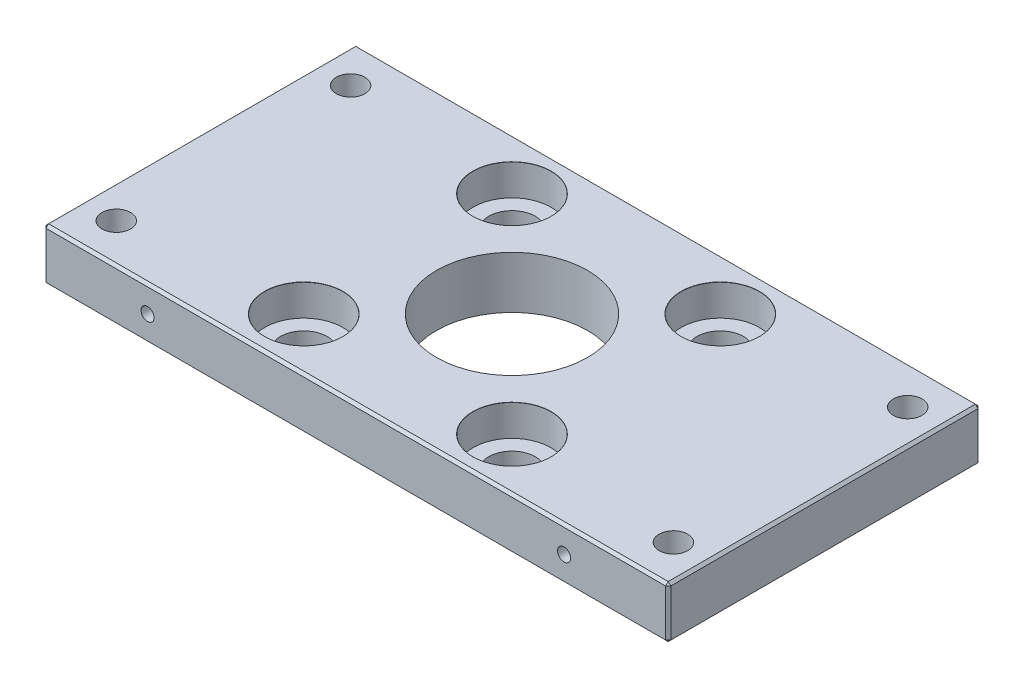
SolidWorks part; units mm, degrees
ref_plane "Front Plane" through (0, 0, 0) normal (0, 0, 1) x (1, 0, 0)
ref_plane "Top Plane" through (0, 0, 0) normal (0, 1, 0) x (1, 0, 0)
ref_plane "Right Plane" through (0, 0, 0) normal (1, 0, 0) x (0, 0, -1)
other "Configuration Table"
sketch "Sketch1" plane through (0, 0, 0) normal (0, 1, 0) x (1, 0, 0)
  line L1 (0, 0) -> (120, 0)
  line L2 (0, 0) -> (0, 60)
  line L3 (0, 60) -> (120, 60)
  line L4 (120, 0) -> (120, 60)
  dimension "D1" = 120
  dimension "D2" = 60
extrude "Boss-Extrude1" add sketch "Sketch1" along normal blind 10
sketch "Sketch2" plane through (0, 10, 0) normal (0, 1, 0) x (1, 0, 0)
  line L0 (0, 30) -> (120, 30) construction
  line L1 (0, 60) -> (0, 0) construction
  line L2 (120, 0) -> (120, 60) construction
  line L3 (60, 60) -> (60, 0) construction
  line L4 (120, 60) -> (0, 60) construction
  line L5 (0, 0) -> (120, 0) construction
  circle A0 centre (60, 30) radius 14.5
  dimension "D1" = 29
extrude "Cut-Extrude1" cut sketch "Sketch2" against normal blind 10
sketch "Sketch4" plane through (0, 10, 0) normal (0, 1, 0) x (1, 0, 0)
  line L0 (60, 60) -> (60, 0) construction
  line L1 (120, 60) -> (0, 60) construction
  line L2 (0, 0) -> (120, 0) construction
  line L3 (0, 30) -> (120, 30) construction
  line L4 (0, 60) -> (0, 0) construction
  line L5 (120, 0) -> (120, 60) construction
  point P16 (40, 50)
  point P17 (80, 50)
  point P21 (40, 10)
  point P22 (80, 10)
  dimension "D1" = 40
  dimension "D2" = 20
  dimension "D3" = 40
  dimension "D4" = 20
  dimension "D5" = 20
  dimension "D6" = 20
  dimension "D7" = 20
  dimension "D8" = 20
hole_wizard "CBORE for M8 Slotted cheese head screws1" positions "Sketch4" profile "Sketch5" counterbore size "M8" standard "GB" end condition through all
sketch "Sketch5" plane through (80, 10, -10) normal (1, 0, 0) x (0, 0, 1)
  line L0 (0, 0) -> (0, 10)
  line L1 (0, 10) -> (4.5, 10)
  line L3 (4.5, 10) -> (4.5, 6)
  line L4 (7.5, 6) -> (4.5, 6)
  line L5 (7.5, 6) -> (7.5, 0.025)
  line L6 (7.5, 0.025) -> (7.525, 0)
  line L7 (7.525, 0) -> (0, 0)
  line L8 (-7.5, 0.025) -> (-7.525, 0) construction
  line L11 (0, -6.35) -> (0, 107.95) construction
  dimension "通孔孔直径" = 9
  dimension "通孔孔深度" = 10
  dimension "柱形沉头孔直径" = 15
  dimension "柱形沉头孔深度" = 6
  dimension "近端锥形沉头孔直径" = 15.05
  dimension "近端锥形沉头孔角度" = 90
sketch "Sketch6" plane through (0, 0, 0) normal (0, -1, 0) x (1, 0, 0)
  line L0 (0, -60) -> (0, 0) construction
  line L1 (0, 0) -> (120, 0) construction
  line L2 (6.5, -7.5) -> (6.5, -52.5) construction
  line L3 (120, 0) -> (120, -60) construction
  line L4 (113.5, -7.5) -> (113.5, -52.5) construction
  point P0 (6.5, -7.5)
  point P5 (6.5, -52.5)
  point P7 (113.5, -7.5)
  point P13 (113.5, -52.5)
  dimension "D1" = 6.5
  dimension "D2" = 7.5
  dimension "D4" = 45
  dimension "D5" = 6.5
  dimension "D7" = 45
  dimension "D8" = 107
  dimension "D3" = 2
  dimension "D6" = 2
hole_wizard "CBORE for M5 Slotted cheese head screws1" positions "Sketch6" profile "Sketch7" counterbore size "M5" standard "GB" end condition through all
sketch "Sketch7" plane through (6.5, 0, -7.5) normal (1, 0, 0) x (0, 0, -1)
  line L0 (0, 0) -> (0, 10)
  line L1 (0, 10) -> (2.75, 10)
  line L3 (2.75, 10) -> (2.75, 5.7)
  line L4 (5, 5.7) -> (2.75, 5.7)
  line L5 (5, 5.7) -> (5, 0.025)
  line L6 (5, 0.025) -> (5.025, 0)
  line L7 (5.025, 0) -> (0, 0)
  line L8 (-5, 0.025) -> (-5.025, 0) construction
  line L11 (0, -6.35) -> (0, 107.95) construction
  dimension "通孔孔直径" = 5.5
  dimension "通孔孔深度" = 10
  dimension "柱形沉头孔直径" = 10
  dimension "柱形沉头孔深度" = 5.7
  dimension "近端锥形沉头孔直径" = 10.05
  dimension "近端锥形沉头孔角度" = 90
sketch "Sketch8" plane through (0, 0, 0) normal (0, -1, 0) x (1, 0, 0)
  line L0 (40, -10) -> (80, -50) construction
  line L1 (80, -10) -> (40, -50) construction
  circle A0 centre (43.182, -13.182) radius 2.5
  circle A1 centre (40, -10) radius 4.5 construction
  circle A2 centre (76.818, -13.182) radius 2.5
  circle A3 centre (80, -10) radius 4.5 construction
  circle A4 centre (76.818, -46.818) radius 2.5
  circle A5 centre (80, -50) radius 4.5 construction
  circle A6 centre (43.182, -46.818) radius 2.5
  circle A7 centre (40, -50) radius 4.5 construction
  dimension "D1" = 5
  dimension "D2" = 5
  dimension "D3" = 5
  dimension "D4" = 5
extrude "Cut-Extrude2" [suppressed] cut sketch "Sketch8" against normal blind 10
sketch "Sketch10" plane through (0, 0, 0) normal (0, 0, 1) x (1, 0, 0)
  line L0 (0, 10) -> (0, 0) construction
  line L1 (0, 10) -> (120, 10) construction
  line L2 (120, 10) -> (120, 0) construction
  point P0 (20, 5)
  point P1 (100, 5)
  dimension "D1" = 20
  dimension "D2" = 5
  dimension "D3" = 20
hole_wizard "M3 Tapped Hole1" positions "Sketch10" profile "Sketch11" tap size "M3" standard "GB"
sketch "Sketch11" plane through (20, 5, 0) normal (1, 0, 0) x (0, -1, 0)
  line L0 (0, 0) -> (0, 12.7511)
  line L1 (0, 12.7511) -> (1.25, 12)
  line L2 (1.25, 12) -> (1.25, 0)
  line L5 (1.25, 0) -> (0, 0)
  line L10 (0, 12.7511) -> (-1.25, 12) construction
  line L11 (0, -6.35) -> (0, 107.95) construction
  dimension "螺纹孔钻头直径" = 2.5
  dimension "螺纹孔钻头深度" = 12
  dimension "导头角度" = 118
cosmetic thread "Hole thread1" parameters "D1"=10, "D2"=3
cosmetic thread "Hole thread2" parameters "D1"=10, "D2"=3
chamfer "Chamfer1" distance 0.5 12 edges at (60, 0, 0) (0, 5, 0) (0, 5, -60) (0, 0, -30) (60, 0, -60) (120, 0, -30) (120, 5, 0) (120, 5, -60) (60, 10, -60) (0, 10, -30) (60, 10, 0) (120, 10, -30)
